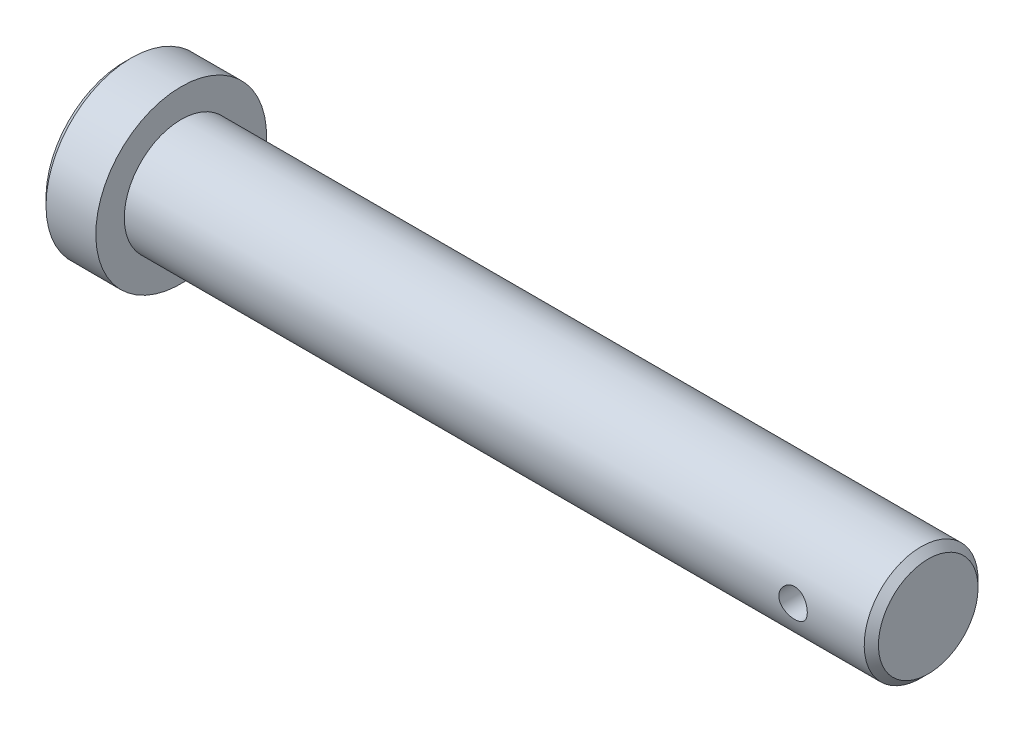
from build123d import *

# Parameters (mm, degrees)
CUT_EXTRUDE1_DEPTH      = 115.267230648
CUT_EXTRUDE1_DEPTH_BACK = 115.267230648
SKETCH2_R               = 2
CHAMFER1_SIZE           = 1
CHAMFER2_SIZE           = 1


with BuildPart() as part:
    # Sketch1 → Revolve1 (revolve)
    with BuildSketch(Plane.XY):
        Polygon((0, 0), (-113, 0), (-113, 12), (-105, 12), (-105, 8), (0, 8), align=None)
    revolve(axis=Axis((0, 0, 0), (-1, 0, 0)))

    # Sketch2 → Cut-Extrude1 (cut, two sides: drawn at the far end of the back side and taken through both)
    with BuildSketch(Plane.XY.offset(-CUT_EXTRUDE1_DEPTH_BACK)):
        with Locations((-11, 0)):
            Circle(SKETCH2_R)
    extrude(amount=CUT_EXTRUDE1_DEPTH + CUT_EXTRUDE1_DEPTH_BACK, mode=Mode.SUBTRACT)

    # Chamfer1
    chamfer1_edges = [part.edges().sort_by_distance(p)[0] for p in [
        (0, -8, 0),
    ]]
    chamfer(chamfer1_edges, length=CHAMFER1_SIZE)

    # Chamfer2
    chamfer2_edges = [part.edges().sort_by_distance(p)[0] for p in [
        (-113, -12, 0),
    ]]
    chamfer(chamfer2_edges, length=CHAMFER2_SIZE)


solid = part.part
